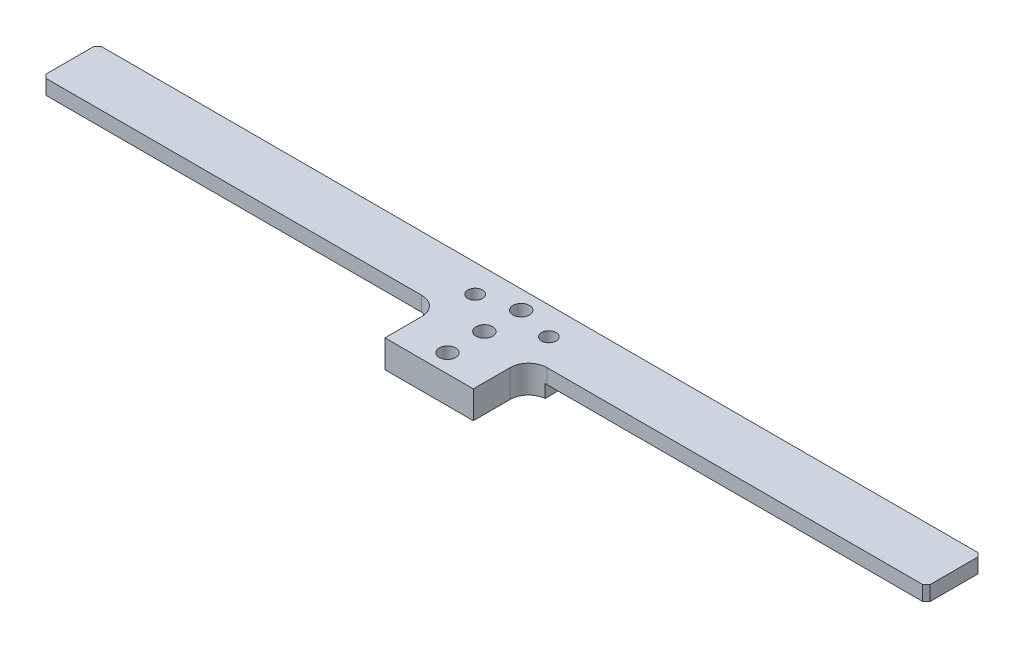
from build123d import *

# Parameters (mm, degrees)
BOSS_EXTRUDE_1_DEPTH   = 4
BOSS_EXTRUDE_2_DEPTH   = 4
FILLET_1_R             = 5
SKETCH_6_W             = 24
SKETCH_6_H             = 30
BOSS_EXTRUDE_3_DEPTH   = 3.5
SKETCH_3_R             = 2.25
CUT_EXTRUDE_1_DEPTH    = 191.738695602
LINEAR_PATTERN_1_COUNT = 3
LINEAR_PATTERN_1_PITCH = 10
SKETCH_7_W             = 63.778369094
SKETCH_7_H             = 56.242484603
CUT_EXTRUDE_2_DEPTH    = 10
CHAMFER_3_SIZE         = 1
SKETCH_8_W             = 4.5
SKETCH_8_H             = 30
BOSS_EXTRUDE_4_DEPTH   = 3.5
CUT_EXTRUDE_START      = -10
CUT_EXTRUDE_3_DEPTH    = 10
F_4_0_4_HOLE_1_D       = 4
LINEAR_PATTERN_2_COUNT = 2
LINEAR_PATTERN_2_PITCH = 20


with BuildPart() as part:
    # Sketch 1 → Boss-Extrude 1 (new body)
    with BuildSketch(Plane.XZ.offset(2)):
        with BuildLine():
            Line((-59, 15), (-69, 15))
            Line((-69, 15), (-70, 15))
            Line((-70, 15), (-70, -15))
            Line((-70, -15), (-69, -15))
            Line((-69, -15), (69, -15))
            Line((69, -15), (70, -14))
            Line((70, -14), (70, -1))
            Line((70, -1), (69, 0))
            Line((69, 0), (-53, 0))
            ThreePointArc((-53, 0), (-56.535533906, 1.464466094), (-58, 5))
            Line((-58, 5), (-58, 15))
            Line((-58, 15), (-59, 15))
        make_face()
    extrude(amount=-BOSS_EXTRUDE_1_DEPTH)

    # Sketch 2 → Boss-Extrude 2 (add)
    with BuildSketch(Plane(origin=(0, 2, 0), x_dir=(1, 0, 0), z_dir=(0, 1, 0))):
        Polygon((-70, 15), (-190, 15), (-190, 0), (-82, 0), (-82, -15), (-70, -15), align=None)
    extrude(amount=-BOSS_EXTRUDE_2_DEPTH)

    # Fillet 1
    fillet_1_edges = [part.edges().sort_by_distance(p)[0] for p in [
        (-82, 0, 0),
    ]]
    fillet(fillet_1_edges, radius=FILLET_1_R)

    # Sketch 6 → Boss-Extrude 3 (add)
    with BuildSketch(Plane.XZ.offset(2)):
        with Locations((-70, 0)):
            Rectangle(SKETCH_6_W, SKETCH_6_H)
    extrude(amount=BOSS_EXTRUDE_3_DEPTH)

    # Sketch 3 → Cut-Extrude 1 (cut, through all)
    with BuildSketch(Plane(origin=(0, 2, 0), x_dir=(1, 0, 0), z_dir=(0, 1, 0))):
        with Locations(Location((-70, -10, 0), (0, 0, 270))):
            Circle(SKETCH_3_R)
    cut_extrude_1 = extrude(amount=-CUT_EXTRUDE_1_DEPTH, mode=Mode.SUBTRACT)

    # Linear Pattern 1: Cut-Extrude 1 ×3
    with Locations(*[(0, 0, -i * LINEAR_PATTERN_1_PITCH) for i in range(1, LINEAR_PATTERN_1_COUNT)]):
        add(cut_extrude_1, mode=Mode.SUBTRACT)

    # Sketch 7 → Cut-Extrude 2 (cut)
    with BuildSketch(Plane(origin=(0, 2, 0), x_dir=(1, 0, 0), z_dir=(0, 1, 0))):
        with Locations((81.889184547, 6.971733155)):
            Rectangle(SKETCH_7_W, SKETCH_7_H)
    extrude(amount=-CUT_EXTRUDE_2_DEPTH, mode=Mode.SUBTRACT)

    # Chamfer 3
    chamfer_3_edges = [part.edges().sort_by_distance(p)[0] for p in [
        (50, 0, -15),
        (50, 0, 0),
        (-190, 0, -15),
        (-190, 0, 0),
    ]]
    chamfer(chamfer_3_edges, length=CHAMFER_3_SIZE)

    # Sketch 8 → Boss-Extrude 4 (add)
    with BuildSketch(Plane.XZ.offset(5.5)):
        with Locations((-55.75, 0)):
            Rectangle(SKETCH_8_W, SKETCH_8_H)
        with Locations((-84.25, 0)):
            Rectangle(SKETCH_8_W, SKETCH_8_H)
    extrude(amount=-BOSS_EXTRUDE_4_DEPTH)

    # Sketch 9 → Cut-Extrude 3 (cut)
    with BuildSketch(Plane(origin=(0, -2, 0), x_dir=(1, 0, 0), z_dir=(0, 1, 0)).offset(CUT_EXTRUDE_START)):
        with BuildLine():
            Line((-53.5, -15), (-58, -15))
            Line((-58, -15), (-58, -5))
            ThreePointArc((-58, -5), (-56.708099244, -1.645898034), (-53.5, -0.025062814))
            Line((-53.5, -0.025062814), (-53.5, -15))
        make_face()
        with BuildLine():
            Line((-82, -15), (-86.5, -15))
            Line((-86.5, -15), (-86.5, -0.025062814))
            ThreePointArc((-86.5, -0.025062814), (-83.291900756, -1.645898034), (-82, -5))
            Line((-82, -5), (-82, -15))
        make_face()
    extrude(amount=CUT_EXTRUDE_3_DEPTH, mode=Mode.SUBTRACT)

    # Ø4.0 (4) Hole 1 (through all)
    with Locations(Plane(origin=(0, 2, 0), x_dir=(-1, 0, 0), z_dir=(0, 1, 0))):
        with Locations((60, -7.5)):
            f_4_0_4_hole_1 = Hole(F_4_0_4_HOLE_1_D / 2)

    # Linear Pattern 2: Ø4.0 (4) Hole 1 ×2
    with Locations(*[(-i * LINEAR_PATTERN_2_PITCH, 0, 0) for i in range(1, LINEAR_PATTERN_2_COUNT)]):
        add(f_4_0_4_hole_1, mode=Mode.SUBTRACT)


solid = part.part
